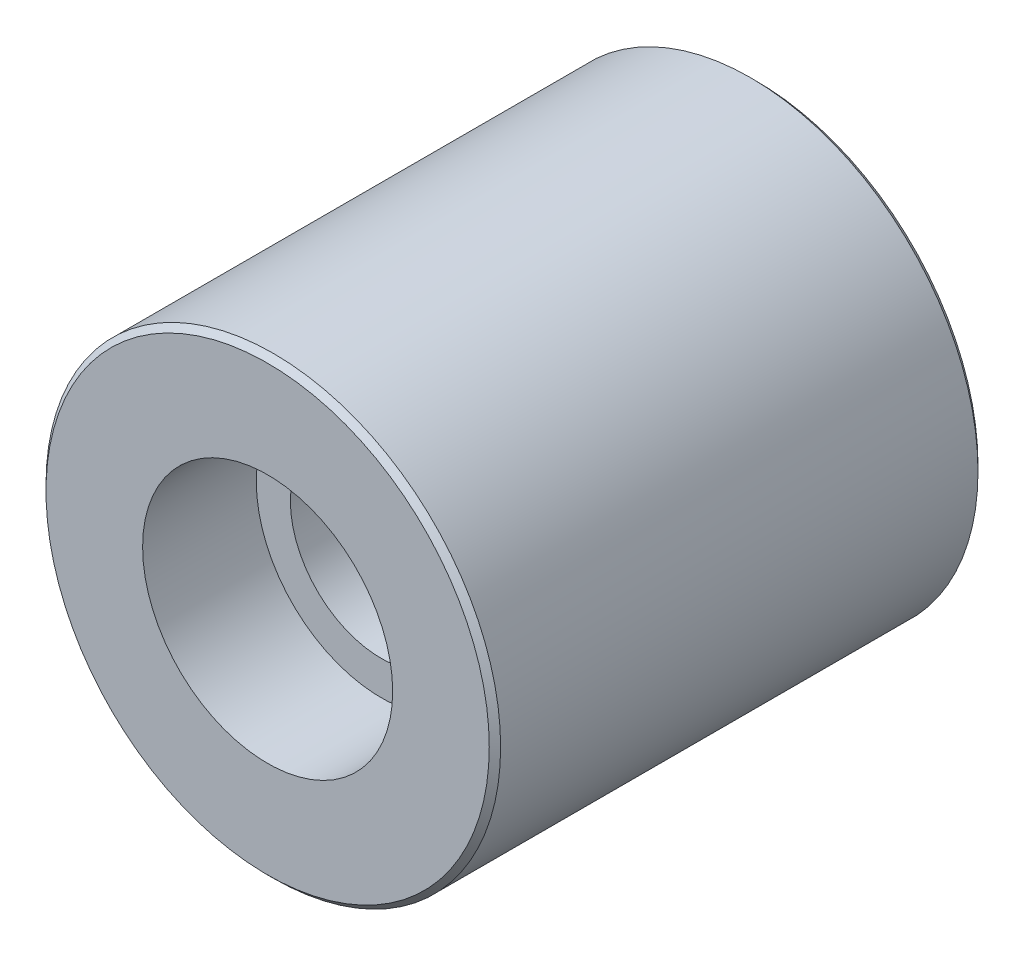
from build123d import *

# Parameters (mm, degrees)
SKETCH_1_R          = 20
EXTRUDE_1_DEPTH     = 43
SKETCH_2_R          = 11
CUT_EXTRUDE_1_DEPTH = 10
CUT_EXTRUDE_START   = -7
SKETCH_3_R          = 11
CUT_EXTRUDE_2_DEPTH = 7
SKETCH_4_R          = 8
CUT_EXTRUDE_3_DEPTH = 46.782092569
CHAMFER_1_SIZE      = 0.5


with BuildPart() as part:
    # 草图1 → 凸台-拉伸1 (new body)
    with BuildSketch(Plane.XY):
        Circle(SKETCH_1_R)
    extrude(amount=EXTRUDE_1_DEPTH)

    # 草图2 → 切除-拉伸1 (cut)
    with BuildSketch(Plane.XY.offset(43)):
        Circle(SKETCH_2_R)
    extrude(amount=-CUT_EXTRUDE_1_DEPTH, mode=Mode.SUBTRACT)

    # 草图3 → 切除-拉伸2 (cut)
    with BuildSketch(Plane(origin=(0, 0, 0), x_dir=(-1, 0, 0), z_dir=(0, 0, -1)).offset(CUT_EXTRUDE_START)):
        with Locations(Location((0, 0, 0), (0, 0, 180))):
            Circle(SKETCH_3_R)
    extrude(amount=CUT_EXTRUDE_2_DEPTH, mode=Mode.SUBTRACT)

    # 草图4 → 切除-拉伸3 (cut, through all)
    with BuildSketch(Plane(origin=(0, 0, 7), x_dir=(-1, 0, 0), z_dir=(0, 0, -1))):
        Circle(SKETCH_4_R)
    extrude(amount=-CUT_EXTRUDE_3_DEPTH, mode=Mode.SUBTRACT)

    # 倒角1
    chamfer_1_edges = [part.edges().sort_by_distance(p)[0] for p in [
        (-20, 0, 0),
        (-20, 0, 43),
    ]]
    chamfer(chamfer_1_edges, length=CHAMFER_1_SIZE)


solid = part.part
